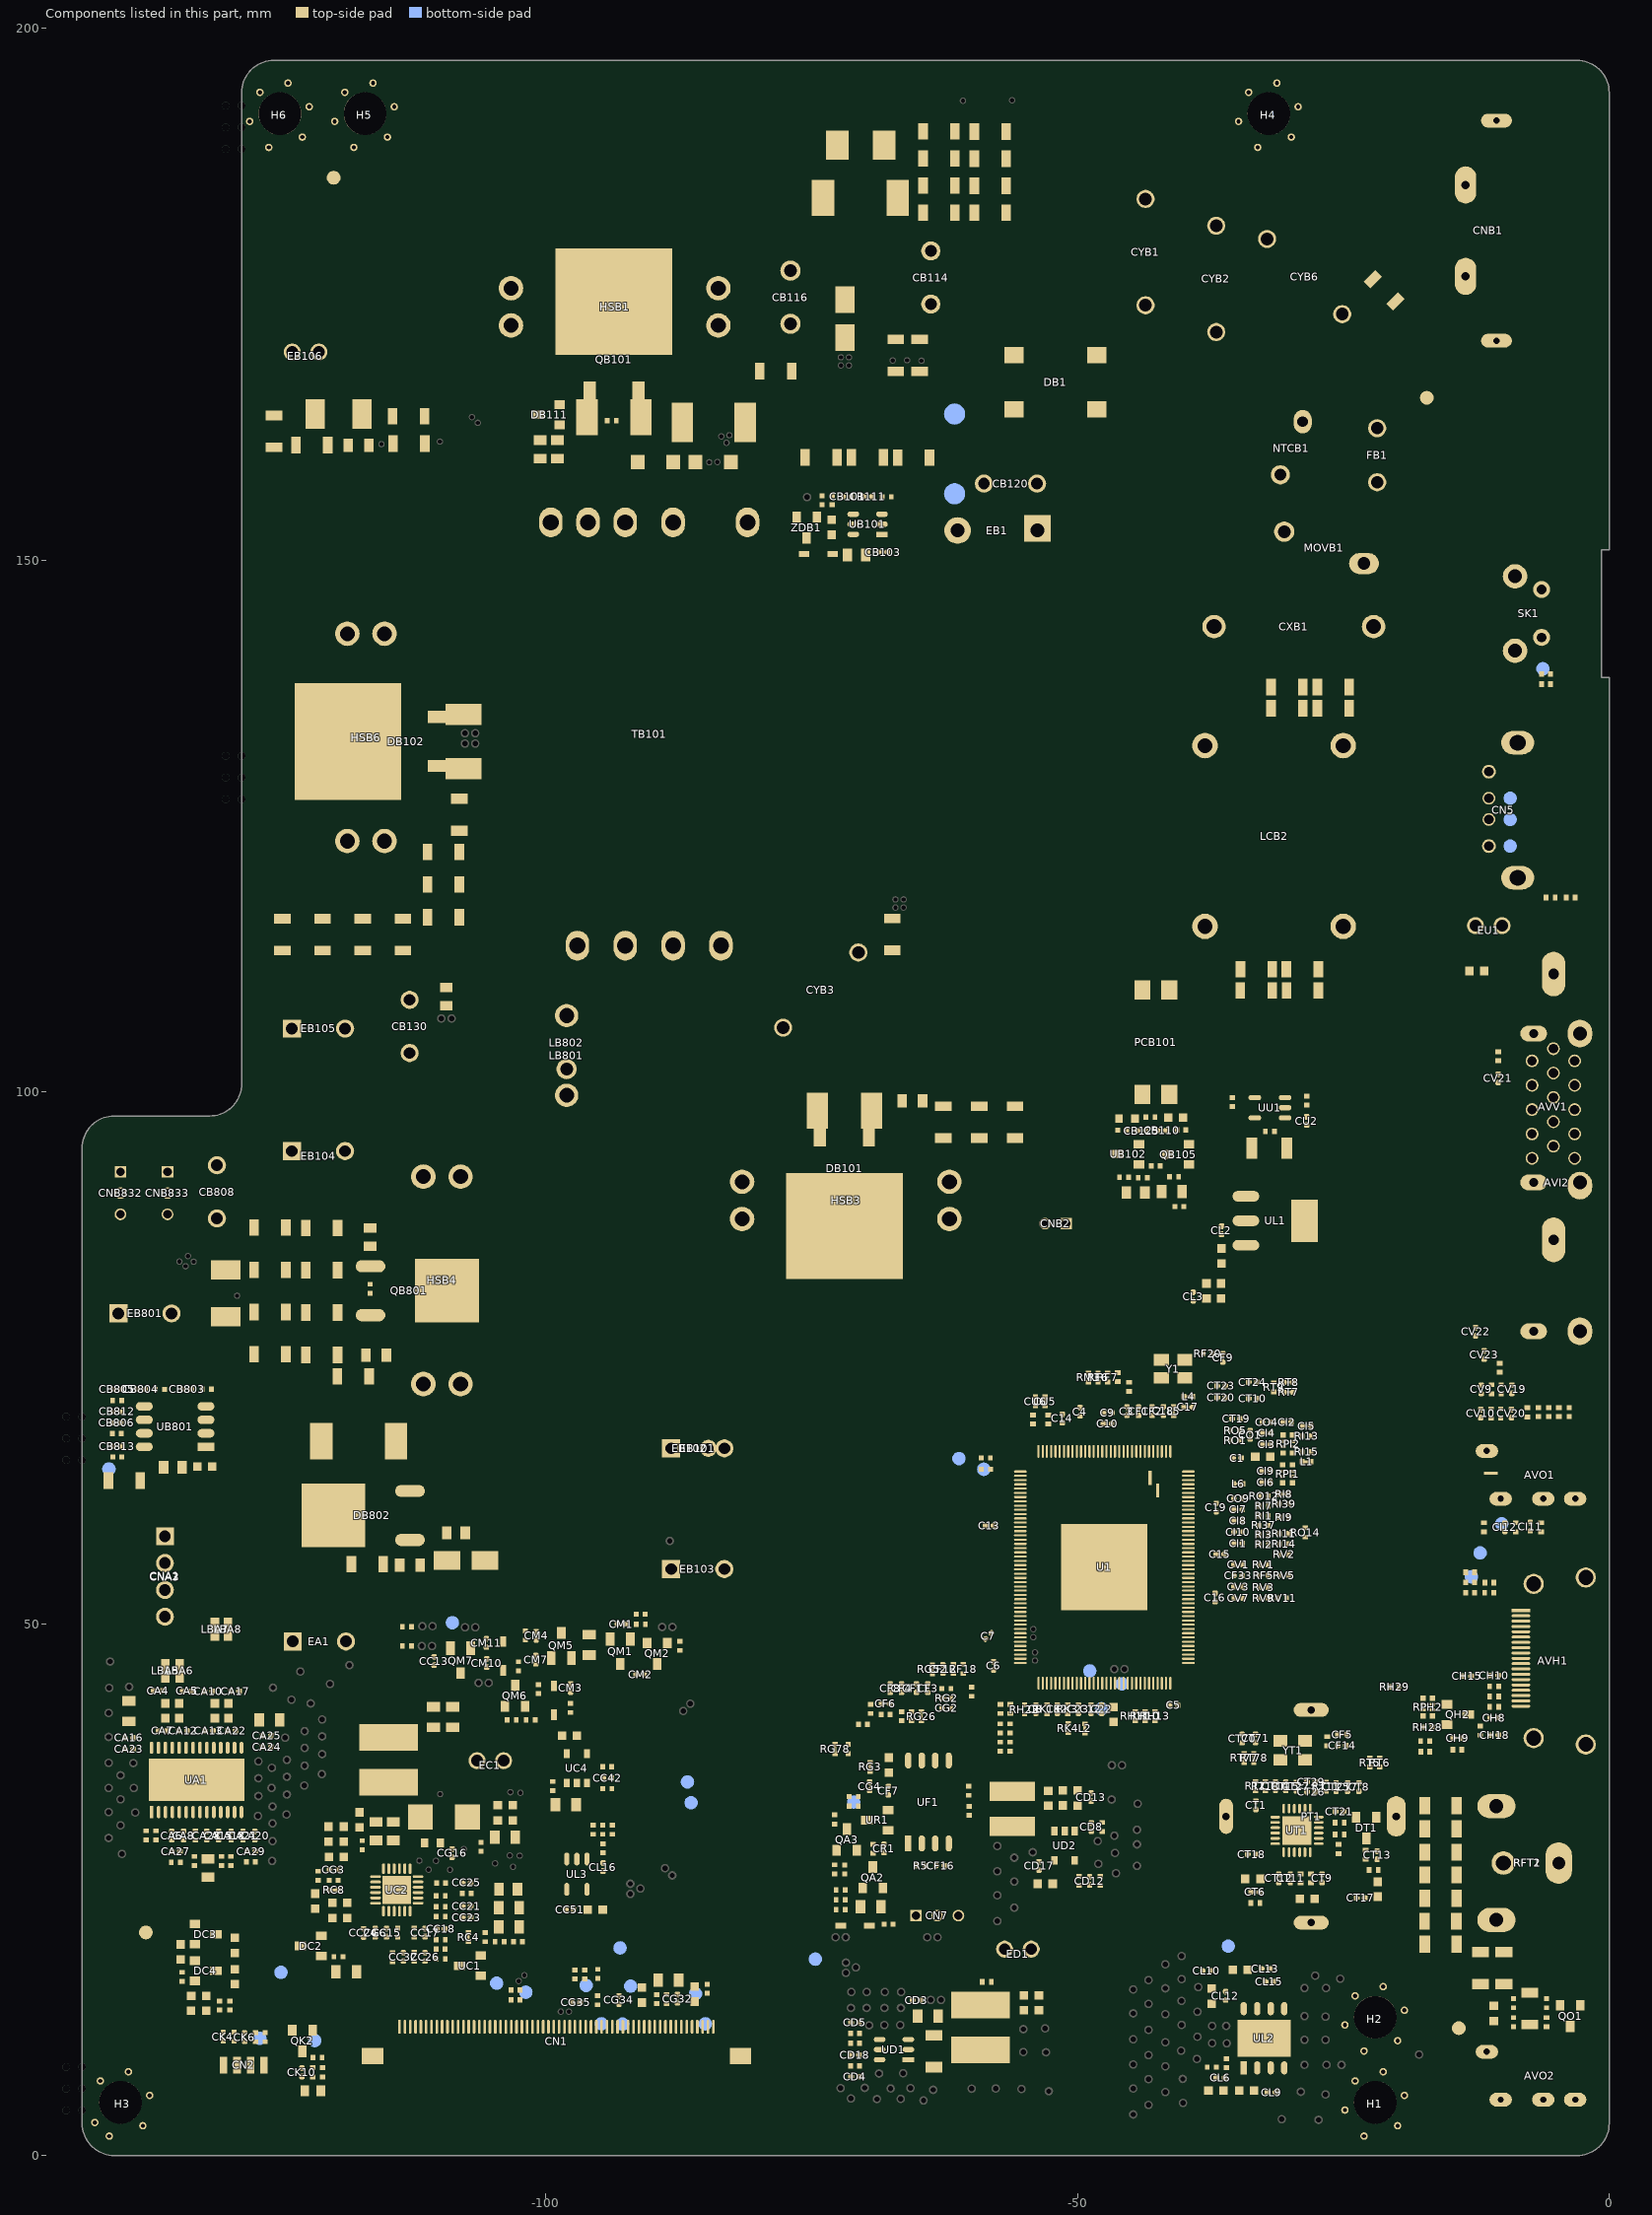
[diagram p0: the components of this part, seen from the top]
# Altium PCB MISC86383-9.PcbDoc (part 18 of 18)
Units mm, origin at the board's own origin, x right, y up, seen from the top; angles counter-clockwise.
Board outline 143.6 x 197 mm, 2 copper layers (TopLayer, BottomLayer), stack 1.571 mm thick; 743 components, 401 nets, 2996 pads, 1077 vias.
Unrouted connection lines stored in the file: 4.

## Silkscreen, mask and mechanical layers (free items; w line width, h text height) (continued)
顶层限制:
  drawing of 20851 lines, arcs and shapes, not listed
  text "Wall-mount position (metal exposed)" at -97.401,250.481 h2.5
  text "Rear housing assembly, slides from right to left; reserve 15mm space" at -97.401,247.956 h2.5
  text "\C2;1) Primary/secondary: height limit H=8.5mm within yellow area;" at -97.401,245.431 h2.5
  text "\C30;2) Primary/secondary: height limit H=1.5mm within orange area." at -97.401,242.906 h2.5
  text "155" at -77.5,223.346 h2.5
  text "128.6" at -64.3,217.346 h2.5
  text "125" at -62.5,211.346 h2.5
  text "No components on top and bottom layers," at -14.151,209.843 h2
  text "routing allowed" at -14.151,207.823 h2
  text "117" at -58.5,205.346 h2.5
  text "4" at -109.474,203.265 h2.5
  text "4" at -103.423,199.984 h2.5
  text "32" at -16,199.346 h2.5
  text "No components on top and bottom layers; routing allowed }" at 1.847,196.017 h2
  text "A}" at -30.017,195.328 h2
  text "B}" at -114.933,190.014 h2
  text "A}" at -124.139,189.934 h2
  text "12" at 121.467,189.8 h2.5 r180
  text "4" at -23.031,184.966 h2.5
  text "AC IN}" at 130.555,182.434 h3
  text "22" at 102.959,179 h2.5 r90
  text "It is recommended that all Y capacitor earths connect to this screw hole," at -64.482,170.89 h2
  text "connecting to the main board ground may seriously affect performance." at -64.482,168.87 h2
  text "No components on top layer; routing allowed }" at 1.847,167.707 h2
  text "4" at 120.442,148.25 h2.5 r180
  text "Within green area," at -55.569,147.272 h2
  text "SWITCH}" at 130.555,146.687 h3
  text "Board shape adjusted per layout }" at -121.928,145.271 h3
  text "front side limits primary components and primary routing" at -55.569,145.252 h2
  text "7.0" at 123.392,143.875 h2.5 r180
  text "7.5" at 108.367,141.85 h2.5 r90
  text "0.7" at 8.179,140.436 h2.5
  text "7.12" at 106.742,138.623 h2.5 r180
  text "0.7" at 8.179,135.33 h2.5
  text "USB IN}" at 130.555,127.629 h3
  text "14.8" at 105.382,124.268 h2.5 r90
  text "Backlight exit }" at -173.323,122.164 h1.5
  text "2.28" at 130.312,119.804 h2.5 r180
  text "1.5" at 9.554,116.806 h2.5
  text "6.3" at 128.251,114.42 h2.5 r180
  text "7.9" at 128.281,111.09 h2.5 r180
  text "10.7" at 180.627,110.448 h2.5 r180
  text "Final position }" at -185.85,108.979 h1.5
  text "Assembly process }" at -171.274,108.979 h1.5
  text "CVBS IN}" at 189.847,106.926 h3
  text "VGA IN}" at 130.555,99.074 h3
  text "197" at 79.231,97.25 h2.5 r90
  text "14" at 11.398,96.717 h2.5 r90
  text "25" at 101.141,96.51 h2.5 r90
  text "192" at 73.231,94.75 h2.5 r90
  text "16.3" at 123.541,94.08 h2.5 r90
  text "CVBS LIN}" at 189.847,93.047 h3
  text "Pay attention to DIP orientation" at -44.734,92.654 h2
  text "LED DRIVER}" at -132.748,91.423 h2
  text "3- 8.3" at 186.942,91.043 h2.5 r150
  text "VGA tinning pad may only be added on the left" at -44.734,90.634 h2
  text "5.2" at 11.19,89.427 h2.5 r90
  text "181" at 67.231,89.25 h2.5 r90
  text "12.6" at 129.516,88.645 h2.5 r180
  text "During rear housing sliding, interference is likely between the backlight harness and the rear housing latch," at -132.931,87.883 h2
  text "40.2" at 157.205,87.512 h2.5 r90
  text "When the upper half is pressed to 128.6mm, place the socket per the structure drawing;" at -132.931,85.863 h2
  text "When the upper half is expanded, place the backlight socket toward the upper left (as close as possible to the backlight exit)." at -132.931,83.843 h2
  text "14" at 11.443,82.717 h2.5 r90
  text "If unsure, ask structure to assess." at -132.931,81.823 h2
  text "CVBS RIN}" at 189.847,79.168 h3
  text "5.5" at 180.471,76.201 h2.5 r180
  text "Maximum board extension area }" at -178.067,73.922 h3
  text "145" at 61.231,71.25 h2.5 r90
  text "5.5" at 125.812,66.794 h2.5 r180
  text "5.5" at 180.436,66.794 h2.5 r180
  text "AV OUT(Mini)}" at 189.847,65.736 h3
  text "AV IN(Mini)}" at 130.555,65.385 h3
  text "5.5" at 105.521,65.003 h2.5 r166
  text "5.5" at 160.144,65.003 h2.5 r166
  text "8" at 122.126,63.594 h2.5 r180
  text "8" at 176.75,63.594 h2.5 r180
  text "126.5" at 55.231,62 h2.5 r90
  text "2" at 8.387,58.551 h2.5
  text "Output on left side of speaker; socket not higher than current position }" at -131.801,58.057 h2
  text "6.25" at 127.988,54.907 h2.5 r180
  text "SPEAKER}" at -131.731,54.033 h2
  text "98.6" at 49.231,48.05 h2.5 r90
  text "HDMI IN}" at 130.555,47.924 h3
  text "15" at 106.692,44.925 h2.5 r90
  text "91.5" at 43.231,44.5 h2.5 r90
  text "9.25" at 128.184,41.064 h2.5 r180
  text "1.5" at 9.554,36.308 h2.5
  text "1) Height limit H=8.5mm within yellow area;" at -58.974,33.975 h2
  text "\C30;2) Height limit H=1.5mm within orange area." at -58.974,31.955 h2
  text "6.3" at 118.642,31.2 h2
  text "64" at 37.231,30.75 h2.5 r90
  text "RF IN}" at 130.555,29.012 h3
  text "11.2" at 102.592,24.175 h2 r90
  text "46.5" at 31.231,22.001 h2.5 r90
  text "10.3" at 5.15,18.503 h2.5
  text "4" at -31.494,17.139 h2.5
  text "B}" at -19.385,16.336 h2
  text "IR}" at -129.448,12.878 h2
  text "LED}" at -124.072,12.844 h2
  text "27.5" at 25.231,12.5 h2.5 r90
  text "4" at -33.092,10.851 h2.5
  text "4" at -150.569,10.823 h2.5
  text "TCON}" at -103.65,10.81 h2
  text "5.5" at 125.812,10.294 h2.5 r180
  text "2" at 8.387,9.944 h2.5
  text "EXT-IR}" at 130.555,9.236 h3
  text "A}" at -138.31,9.193 h2
  text "5.5" at 105.521,8.503 h2.5 r166
  text "8" at 122.126,7.094 h2.5 r180
  text "13" at 19.231,5.25 h2.5 r90
  text "A}" at -18.796,4.364 h2
  text "1.6" at 126.442,-3.851 h2.5
  text "7.5" at 18.992,-4.348 h2.5
  text "22" at -11,-6.692 h2.5
  text "5" at 11.198,-7.79 h2.5
  text "No components on top and bottom layers; routing allowed }" at -29.995,-10.289 h2
  text "No components on top and bottom layers; routing allowed }" at 2.218,-10.289 h2
  text "99" at -49.5,-12.692 h2.5
  text "121.9" at -60.95,-18.692 h2.5
  text "1) Height limit H=8.5mm within yellow area;" at -184.708,-22.74 h2
  text "128.4" at -64.2,-24.692 h2.5
  text "\C30;2) Height limit H=1.5mm within orange area." at -184.708,-24.76 h2
  text "140" at -70,-30.692 h2.5
  text "143.6" at -71.8,-36.692 h2.5
  text "145" at -72.5,-42.692 h2.5
  text "2.2" at -129.607,-60.49 h1.27
  text "R1.3" at -129.295,-67.485 h1.27
  text "1.8" at -124.154,-69.06 h1.27 r90
  text "1.6" at -2.688,-72.473 h2.5
底层限制:
  circle w0.127: c403.948,6.341 r2.5
  circle w0.127: c-32,192 r17
  circle w0.127: c-140,5 r2
  circle w0.127: c-32,192 r7
  circle w0.127: c-140,5 r7
  circle w0.127: c-140,5 r9.5
  circle w0.127: c-32,192 r19
  circle w0.127: c-32,192 r9.5
  circle w0.127: c-117,192 r2
  circle w0.127: c-125,192 r2
  circle w0.127: c-22,5 r2
  circle w0.127: c-22,13 r2
  circle w0.127: c-32,192 r2
  lines w0.127: -7.634,-9.254 -2.864,1.63 ; -7.583,201.938 -4.43,195.974 ; -3.661,0 0,0 0,4.754 ; -140.6,0 cw(c-140.6,3) -143.6,3 -143.6,94.75 cw(c-140.6,94.75) -140.6,97.75 -131.6,97.75 ccw(c-131.6,100.75) -128.6,100.75 -128.6,194 cw(c-125.6,194) -125.6,197 ; -140.6,0 -3,0 ccw(c-3,3) 0,3 0,139 -0.7,139 -0.7,151 0,151 0,194 ccw(c-3,194) -3,197 -125.6,197 ; -140.6,0 -142,0 cw(c-142,3) -145,3 -145,96.25 ccw(c-148,96.25) -148,99.25 -152,99.25 cw(c-152,102.25) -155,102.25 -155,194 cw(c-152,194) -152,197 -125.6,197 ; -9,193.5 -9,195 ; -9,193.5 0,193.5 ; -9,193.5 -9,195 ; -9,193.5 0,193.5 ; -9,193.5 -9,195 ; -9,193.5 0,193.5 ; -9,195 0,195 ; -9,195 0,195 ; -9,195 0,195 ; 0,193.5 0,195 ; 0,193.5 0,195 ; -125,173 cw(c-125,192) -125,211 -117,211 cw(c-117,192) -117,173 -125,173 ; -125,175 cw(c-125,192) -125,209 -117,209 cw(c-117,192) -117,175 -125,175 ; -125,182.5 cw(c-125,192) -125,201.5 -117,201.5 cw(c-117,192) -117,182.5 -125,182.5 ; -125,185 cw(c-125,192) -125,199 -117,199 cw(c-117,192) -117,185 -125,185 ; -31.5,5 ccw(c-22,5) -12.5,5 -12.5,13 ccw(c-22,13) -31.5,13 -31.5,5 ; -29,5 ccw(c-22,5) -15,5 -15,13 ccw(c-22,13) -29,13 -29,5 ; -9,2 -9,3.5 0,3.5 0,2 -9,2
附加说明:
  region: -130.1,194 -128.6,194 -128.6,187.42 -130.1,187.42 hole: -129.35,190.426 -129.634,190.71 -129.35,190.994 -129.066,190.71
  region: -130.1,132.865 -128.6,132.865 -128.6,126.285 -130.1,126.285 hole: -129.35,129.291 -129.634,129.575 -129.35,129.859 -129.066,129.575
  region: -143.6,64.135 -145.1,64.135 -145.1,70.715 -143.6,70.715 hole: -144.35,67.709 -144.066,67.425 -144.35,67.141 -144.634,67.425
  region: -143.6,3 -145.1,3 -145.1,9.58 -143.6,9.58 hole: -144.35,6.574 -144.066,6.29 -144.35,6.006 -144.634,6.29
  lines w0.127: 184.316,150.38 213.018,150.38 ; 184.316,153.107 213.018,153.107 ; 184.316,155.833 213.018,155.833 ; 184.316,158.559 213.018,158.559 ; 184.316,161.285 220.65,161.285 ; 191.948,147.654 191.948,164.012 ; 213.018,147.654 213.018,164.012 ; 221.997,150.38 271.997,150.38 ; 221.997,153.107 271.997,153.107 ; 221.997,155.833 271.997,155.833 ; 221.997,158.559 271.997,158.559 ; 221.997,161.285 271.997,161.285 ; 224.651,147.654 224.651,161.285 ; 184.316,147.654 184.316,164.012 220.65,164.012 220.65,147.654 184.316,147.654 ; 221.997,147.654 271.997,147.654 271.997,164.012 221.997,164.012 221.997,147.654
  text "Keep the description brief so derived projects or board revisions can inherit it:" at 232.267,162.869 h0.89
  text "Version cycle number" at 184.871,162.154 h1.52
  text "Customer" at 215.82,162.154 h1.52
  text "Special notes" at 222.793,162.154 h1.52
  text "PCB designer" at 198.98,162.141 h1.52
  text "Template date:" at 147.888,162.082 h1.52
  text "2019.12.06" at 156.067,161.993 h1.52
  text "For new or special design rules: hole spacing for the Bangladesh region; special safety clearance; special stackup not allowed to change; support chain; designated factory..." at 232.254,161.713 h0.89
  text "Material utilization:" at 147.875,159.618 h1.52
  text "8X%" at 156.067,159.516 h1.52
  text "(Fill in for non-TV division projects)" at 160.893,159.516 h1.52
  text "XXXXXX" at 185.366,159.436 h1.52
  text "1" at 223.047,159.436 h1.52
  text "CH & CHJ" at 193.087,159.415 h1.52
  text "2" at 223.045,156.714 h1.52
  text "COMPANY_A" at 214.017,154.093 h1.52
  text "3" at 223.047,153.996 h1.52
  text "4" at 223.047,151.253 h1.52
  text "① Panel production, single-board shipment" at 133.512,150.271 h0.76
  text "Fabrication special requirements; leave blank if none;" at 112.078,149.441 h1.52
  text "Reference:" at 130.083,149.42 h1.52
  text "② 4-up panel production, 2-up panel shipment" at 133.499,149.153 h0.76
  text "5" at 223.047,148.535 h1.52
  text "Copy the notes below to the TopOverlay layer; one or two items may be noted" at 137.411,83.888 h1.52
  text "Only one barcode position on board; the other barcode goes on a component" at 175.984,83.814 h1.52
  text "SMD parts 3.5mm from PCB rail edge; production needs special control" at 119.504,81.805 h1.52
  text "No barcode position on board; barcode goes on a component" at 175.984,81.802 h1.52
  text "Customer special requirements; special process requirements; leave blank if none" at 119.454,78.936 h1.52
  text "Height and designators of SMD parts over 2mm on solder side; leave blank if none" at 119.454,76.396 h1.52
  text "Easily damaged component designators; leave blank if none" at 119.409,72.683 h1.52
  text "New footprint designators; leave blank if none" at 119.469,67.424 h1.52
  text "Suction cup and press pin positions reserved: enter \"Yes\", otherwise \"No\"" at 119.491,62.272 h1.52
  text "X.XXXX.XXX Stencil Revision Explanation" at 96.015,13.731 h1.52
  text "X.XXXX.XXX Testing jig Revision Explanation" at 96.002,11.978 h1.52
  text "X.XXXX.XXX Wave-soldering jig Revision Explanation" at 95.99,10.251 h1.52
DrillDrawing:
  text ".Legend" at 96.144,165.135 h1.52